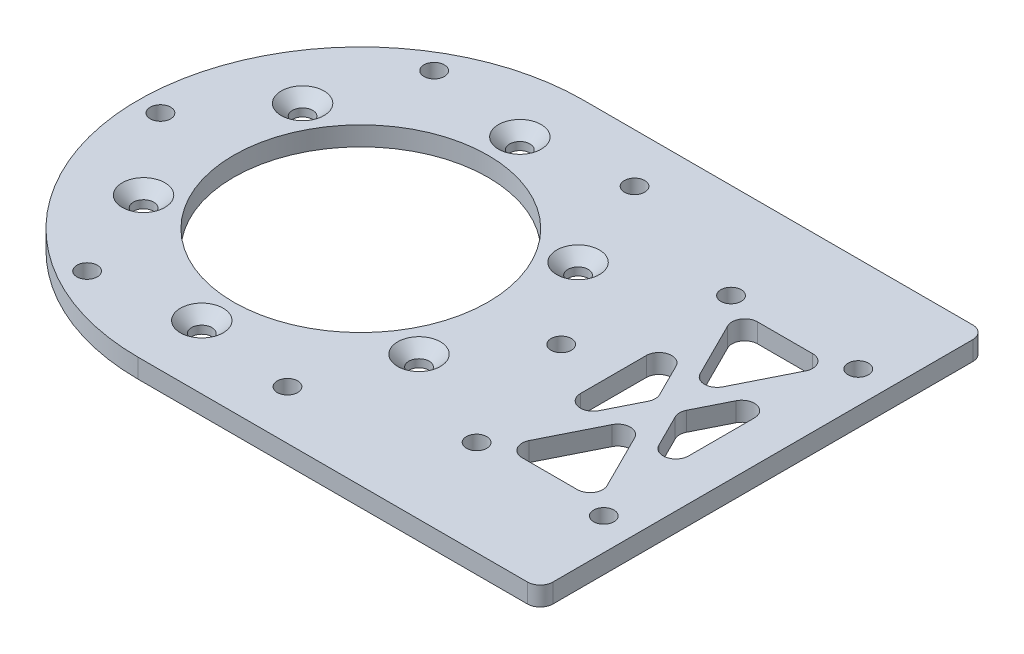
from build123d import *

# Parameters (mm, degrees)
SKETCH_1_R                  = 1.6
SKETCH_1_R_2                = 20
EXTRUDE_1_DEPTH             = 3
HOLE_WIZARD_M3_1_AT_2_COUNT = 2
HOLE_WIZARD_M3_1_AT_2_PITCH = 25
HOLE_WIZARD_M3_1_AT_3_COUNT = 2
HOLE_WIZARD_M3_1_AT_3_PITCH = 43.301270189
HOLE_WIZARD_M3_1_AT_4_COUNT = 2
HOLE_WIZARD_M3_1_AT_4_PITCH = 50
HOLE_WIZARD_M3_1_AT_5_COUNT = 2
HOLE_WIZARD_M3_1_AT_5_PITCH = 43.301270189
HOLE_WIZARD_M3_1_AT_6_COUNT = 2
HOLE_WIZARD_M3_1_AT_6_PITCH = 25
SKETCH_3_R                  = 1.6
CUT_EXTRUDE_1_DEPTH         = 10
CUT_EXTRUDE_2_DEPTH         = 10
FILLET_1_R                  = 2


with BuildPart() as part:
    # 草图1 → 凸台-拉伸1 (new body)
    with BuildSketch(Plane(origin=(0, 0, 0), x_dir=(1, 0, 0), z_dir=(0, 1, 0))):
        with BuildLine():
            Line((-63.2, 35), (0, 35))
            Line((0, 35), (0, -35))
            Line((0, -35), (-63.2, -35))
            ThreePointArc((-63.2, -35), (-98.2, 0), (-63.2, 35))
        make_face()
        with Locations(Location((-63.2, 25, 0), (0, 0, 270))):
            Circle(SKETCH_1_R, mode=Mode.SUBTRACT)
        with Locations(Location((-41.549364905, 12.5, 0), (0, 0, 270))):
            Circle(SKETCH_1_R, mode=Mode.SUBTRACT)
        with Locations(Location((-41.549364905, -12.5, 0), (0, 0, 270))):
            Circle(SKETCH_1_R, mode=Mode.SUBTRACT)
        with Locations(Location((-63.2, -25, 0), (0, 0, 270))):
            Circle(SKETCH_1_R, mode=Mode.SUBTRACT)
        with Locations(Location((-84.850635095, -12.5, 0), (0, 0, 270))):
            Circle(SKETCH_1_R, mode=Mode.SUBTRACT)
        with Locations(Location((-84.850635095, 12.5, 0), (0, 0, 270))):
            Circle(SKETCH_1_R, mode=Mode.SUBTRACT)
        with Locations(Location((-63.2, 0, 0), (0, 0, 270))):
            Circle(SKETCH_1_R_2, mode=Mode.SUBTRACT)
        with Locations(Location((-25, 20, 0), (0, 0, 270))):
            Circle(SKETCH_1_R, mode=Mode.SUBTRACT)
        with Locations(Location((-5, 20, 0), (0, 0, 270))):
            Circle(SKETCH_1_R, mode=Mode.SUBTRACT)
        with Locations(Location((-5, -20, 0), (0, 0, 270))):
            Circle(SKETCH_1_R, mode=Mode.SUBTRACT)
        with Locations(Location((-25, -20, 0), (0, 0, 270))):
            Circle(SKETCH_1_R, mode=Mode.SUBTRACT)
    extrude(amount=EXTRUDE_1_DEPTH)

    # 草图2 → M3 六角凹锥坑螺钉的锥形沉头孔1 (revolve, cut)
    with BuildSketch(Plane(origin=(-63.2, 3, -25), x_dir=(0, 0, 1), z_dir=(1, 0, 0))):
        Polygon((0, 0), (0, 3), (1.6, 3), (1.6, 1.76), (3.36, 0), align=None)
    hole_wizard_m3_1 = revolve(axis=Axis((-63.2, 9.35, -25), (0, -1, 0)), mode=Mode.SUBTRACT)

    # M3 六角凹锥坑螺钉的锥形沉头孔1 at 2: M3 六角凹锥坑螺钉的锥形沉头孔1 ×2
    with Locations(*[Vector(0.8660254037844387, 0, 0.5) * (i * HOLE_WIZARD_M3_1_AT_2_PITCH) for i in range(1, HOLE_WIZARD_M3_1_AT_2_COUNT)]):
        add(hole_wizard_m3_1, mode=Mode.SUBTRACT)

    # M3 六角凹锥坑螺钉的锥形沉头孔1 at 3: M3 六角凹锥坑螺钉的锥形沉头孔1 ×2
    with Locations(*[Vector(0.5000000000000001, 0, 0.8660254037844386) * (i * HOLE_WIZARD_M3_1_AT_3_PITCH) for i in range(1, HOLE_WIZARD_M3_1_AT_3_COUNT)]):
        add(hole_wizard_m3_1, mode=Mode.SUBTRACT)

    # M3 六角凹锥坑螺钉的锥形沉头孔1 at 4: M3 六角凹锥坑螺钉的锥形沉头孔1 ×2
    with Locations(*[(0, 0, i * HOLE_WIZARD_M3_1_AT_4_PITCH) for i in range(1, HOLE_WIZARD_M3_1_AT_4_COUNT)]):
        add(hole_wizard_m3_1, mode=Mode.SUBTRACT)

    # M3 六角凹锥坑螺钉的锥形沉头孔1 at 5: M3 六角凹锥坑螺钉的锥形沉头孔1 ×2
    with Locations(*[Vector(-0.49999999999999983, 0, 0.8660254037844388) * (i * HOLE_WIZARD_M3_1_AT_5_PITCH) for i in range(1, HOLE_WIZARD_M3_1_AT_5_COUNT)]):
        add(hole_wizard_m3_1, mode=Mode.SUBTRACT)

    # M3 六角凹锥坑螺钉的锥形沉头孔1 at 6: M3 六角凹锥坑螺钉的锥形沉头孔1 ×2
    with Locations(*[Vector(-0.8660254037844388, 0, 0.4999999999999997) * (i * HOLE_WIZARD_M3_1_AT_6_PITCH) for i in range(1, HOLE_WIZARD_M3_1_AT_6_COUNT)]):
        add(hole_wizard_m3_1, mode=Mode.SUBTRACT)

    # 草图3 → 切除-拉伸1 (cut)
    with BuildSketch(Plane(origin=(0, 3, 0), x_dir=(1, 0, 0), z_dir=(0, 1, 0))):
        with Locations(Location((-31.7, 0, 0), (0, 0, 270))):
            Circle(SKETCH_3_R)
        with Locations(Location((-47.45, -27.279800219, 0), (0, 0, 270))):
            Circle(SKETCH_3_R)
        with Locations(Location((-78.95, -27.279800219, 0), (0, 0, 270))):
            Circle(SKETCH_3_R)
        with Locations(Location((-94.7, 0, 0), (0, 0, 270))):
            Circle(SKETCH_3_R)
        with Locations(Location((-78.95, 27.279800219, 0), (0, 0, 270))):
            Circle(SKETCH_3_R)
        with Locations(Location((-47.45, 27.279800219, 0), (0, 0, 270))):
            Circle(SKETCH_3_R)
    extrude(amount=-CUT_EXTRUDE_1_DEPTH, mode=Mode.SUBTRACT)

    # 草图4 → 切除-拉伸2 (cut)
    with BuildSketch(Plane(origin=(0, 3, 0), x_dir=(1, 0, 0), z_dir=(0, 1, 0))):
        Polygon((-23.5, 13.645898034), (-23.5, -13.645898034), (-16.677050983, 0), align=None)
        Polygon((-15, -3.354101966), (-22.572949017, -18.5), (-7.427050983, -18.5), align=None)
        Polygon((-7.427050983, 18.5), (-22.572949017, 18.5), (-15, 3.354101966), align=None)
        Polygon((-13.322949017, 0), (-6.5, -13.645898034), (-6.5, 13.645898034), align=None)
    extrude(amount=-CUT_EXTRUDE_2_DEPTH, mode=Mode.SUBTRACT)

    # 圆角1
    fillet_1_edges = [part.edges().sort_by_distance(p)[0] for p in [
        (-22.572949017, 1.5, 18.5),
        (-15, 1.5, 3.354101966),
        (-7.427050983, 1.5, 18.5),
        (-22.572949017, 1.5, -18.5),
        (-7.427050983, 1.5, -18.5),
        (-15, 1.5, -3.354101966),
        (-13.322949017, 1.5, 0),
        (-6.5, 1.5, -13.645898034),
        (-6.5, 1.5, 13.645898034),
        (-23.5, 1.5, 13.645898034),
        (-23.5, 1.5, -13.645898034),
        (-16.677050983, 1.5, 0),
        (0, 1.5, -35),
        (0, 1.5, 35),
    ]]
    fillet(fillet_1_edges, radius=FILLET_1_R)


solid = part.part
